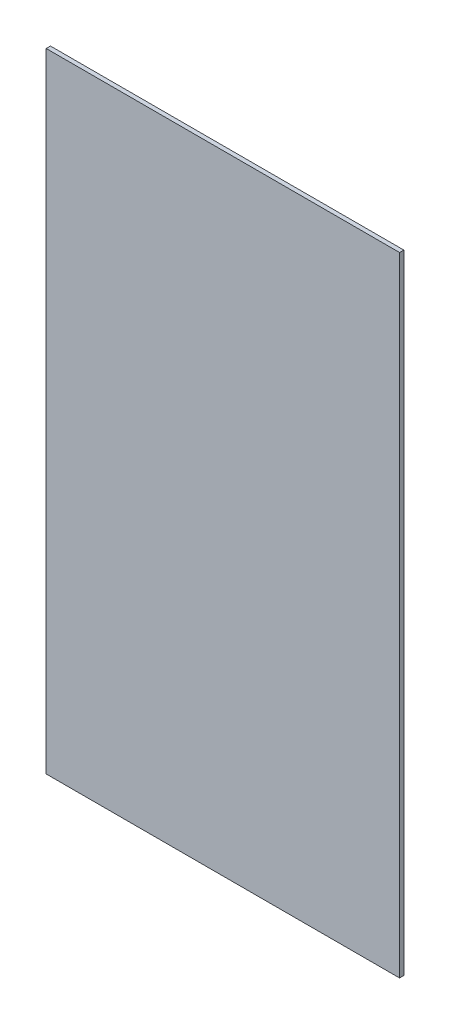
from build123d import *

# Parameters (mm, degrees)
SKETCH_1_W      = 414
SKETCH_1_H      = 736
EXTRUDE_1_DEPTH = 5


with BuildPart() as part:
    # 草图1 → 凸台-拉伸1 (new body)
    with BuildSketch(Plane.XY):
        Rectangle(SKETCH_1_W, SKETCH_1_H)
    extrude(amount=EXTRUDE_1_DEPTH)


solid = part.part
